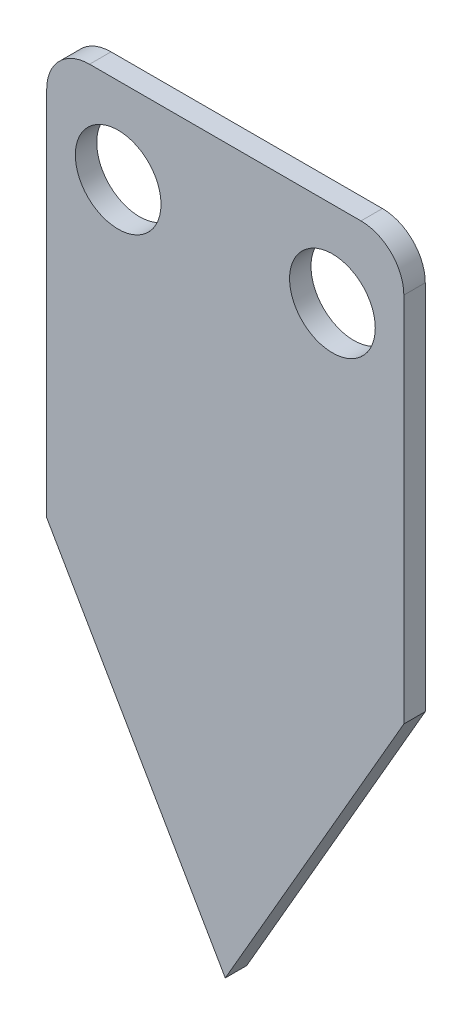
from build123d import *

# Parameters (mm, degrees)
EXTRUDE_1_DEPTH       = 1.5
HOLE_WIZARD_6_0_6_1_D = 6
FILLET_1_R            = 3


with BuildPart() as part:
    # 草图1 → 凸台-拉伸1 (new body)
    with BuildSketch(Plane.XY):
        Polygon((-12.5, 0), (12.5, 0), (12.5, -29), (0, -50.650635095), (-12.5, -29), align=None)
    extrude(amount=EXTRUDE_1_DEPTH)

    # Ø6.0 (6) 直径孔1 (through all)
    with Locations(Plane.XY.offset(1.5)):
        with Locations((-7.5, -6), (7.5, -6)):
            Hole(HOLE_WIZARD_6_0_6_1_D / 2)

    # 圆角1
    fillet_1_edges = [part.edges().sort_by_distance(p)[0] for p in [
        (-12.5, 0, 0.75),
        (12.5, 0, 0.75),
    ]]
    fillet(fillet_1_edges, radius=FILLET_1_R)


solid = part.part
